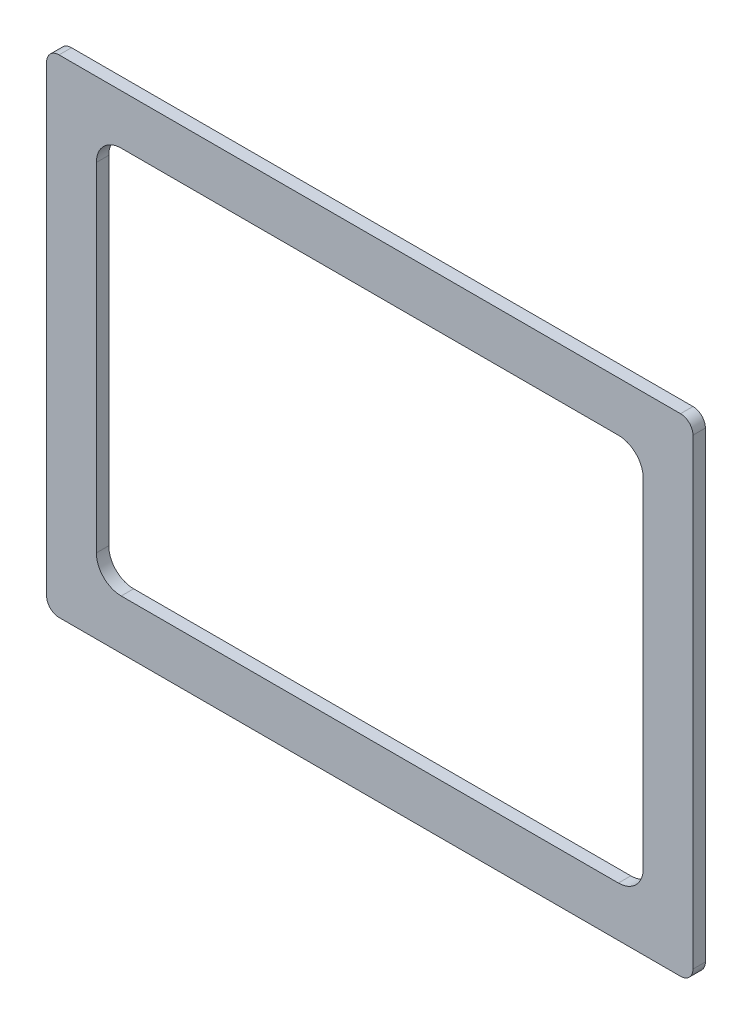
SolidWorks part; units mm, degrees
material "Plain Carbon Steel"
ref_plane "Front Plane" through (0, 0, 0) normal (0, 0, 1) x (1, 0, 0)
ref_plane "Top Plane" through (0, 0, 0) normal (0, 1, 0) x (1, 0, 0)
ref_plane "Right Plane" through (0, 0, 0) normal (1, 0, 0) x (0, 0, -1)
sketch "Sketch1" plane through (0, 0, 0) normal (0, 0, 1) x (1, 0, 0)
  line L0 (0, -4190.1927) -> (0, 205319.4418) construction
  line L1 (-4190.1927, 0) -> (205319.4418, 0) construction
  line L2 (-110, 78) -> (110, 78)
  line L3 (-130, 98) -> (130, 98)
  line L4 (-130, 98) -> (-130, -98)
  line L5 (-130, -98) -> (130, -98)
  line L6 (130, 98) -> (130, -98)
  line L7 (110, 78) -> (110, -78)
  line L8 (-110, -78) -> (110, -78)
  line L9 (-110, 78) -> (-110, -78)
  dimension "D1" = 260
  dimension "D2" = 196
  dimension "D3" = 20
extrude "Boss-Extrude1" add sketch "Sketch1" along normal blind 5
fillet "Fillet1" radius 5 4 edges at (130, 98, 2.5) (130, -98, 2.5) (-130, -98, 2.5) (-130, 98, 2.5)
fillet "Fillet2" radius 10 4 edges at (110, 78, 2.5) (-110, 78, 2.5) (-110, -78, 2.5) (110, -78, 2.5)
